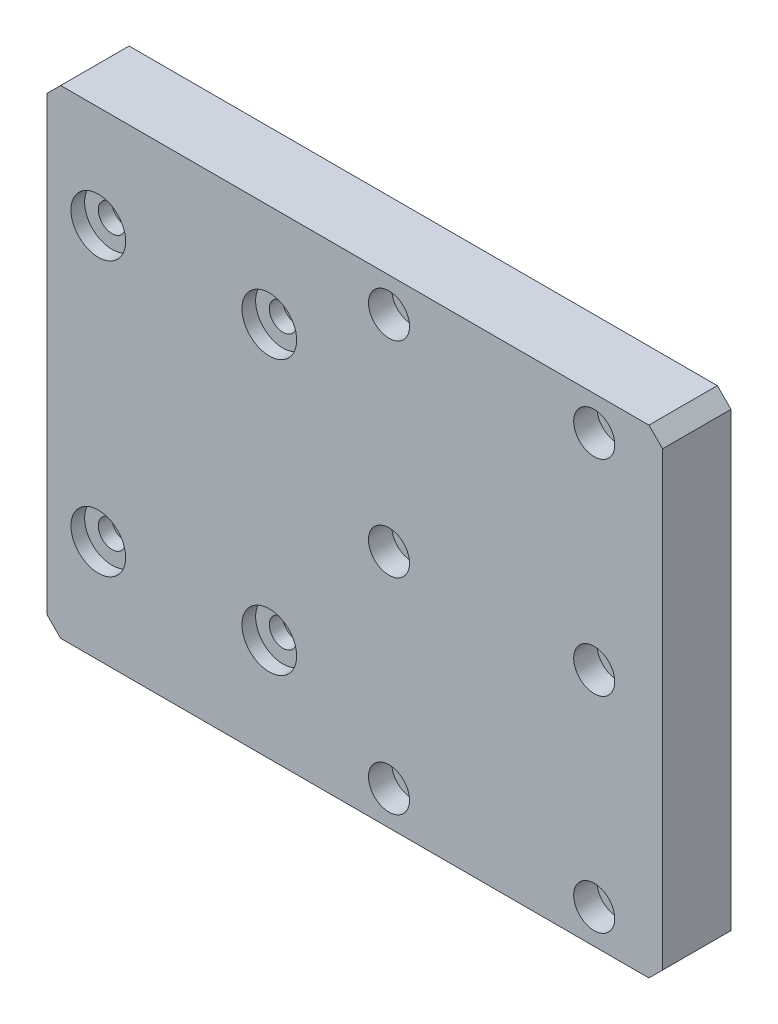
from build123d import *

# Parameters (mm, degrees)
SKETCH_1_W                = 90
SKETCH_1_H                = 70
EXTRUDE_1_DEPTH           = 5
HOLE_WIZARD_1_D           = 3.4
HOLE_WIZARD_1_CBORE_D     = 6
HOLE_WIZARD_1_CBORE_DEPTH = 3.4
HOLE_WIZARD_3_D           = 3.2
HOLE_WIZARD_3_CBORE_D     = 6
HOLE_WIZARD_3_CBORE_DEPTH = 3.4
SKETCH_6_R                = 4
CUT_EXTRUDE_1_DEPTH       = 2
SKETCH_8_R                = 2
CUT_EXTRUDE_2_DEPTH       = 2
CHAMFER_1_SIZE            = 2


with BuildPart() as part:
    # 草图1 → 凸台-拉伸1 (new, symmetric)
    with BuildSketch(Plane.XY):
        Rectangle(SKETCH_1_W, SKETCH_1_H)
    extrude(amount=EXTRUDE_1_DEPTH, both=True)

    # 打孔尺寸(%根据)内六角圆柱头螺钉的类型1 (through all)
    with Locations(Plane.XY.offset(5)):
        with Locations((5, 30), (5, 0), (5, -30), (35, 30), (35, 0), (35, -30)):
            CounterBoreHole(HOLE_WIZARD_1_D / 2, HOLE_WIZARD_1_CBORE_D / 2, HOLE_WIZARD_1_CBORE_DEPTH)

    # 打孔尺寸(%根据)内六角圆柱头螺钉的类型3 (through all)
    with Locations(Plane(origin=(0, 0, -5), x_dir=(-1, 0, 0), z_dir=(0, 0, -1))):
        with Locations((37.5, 20), (12.5, 20), (12.5, -20), (37.5, -20)):
            CounterBoreHole(HOLE_WIZARD_3_D / 2, HOLE_WIZARD_3_CBORE_D / 2, HOLE_WIZARD_3_CBORE_DEPTH)

    # 草图6 → 切除-拉伸1 (cut)
    with BuildSketch(Plane.XY.offset(5)):
        with Locations((-37.5, 20)):
            Circle(SKETCH_6_R)
        with Locations((-12.5, 20)):
            Circle(SKETCH_6_R)
        with Locations((-37.5, -20)):
            Circle(SKETCH_6_R)
        with Locations((-12.5, -20)):
            Circle(SKETCH_6_R)
    extrude(amount=-CUT_EXTRUDE_1_DEPTH, mode=Mode.SUBTRACT)

    # 草图8 → 切除-拉伸2 (cut)
    with BuildSketch(Plane.XY.offset(3)):
        with Locations((-37.5, 20)):
            Circle(SKETCH_8_R)
        with Locations((-37.5, -20)):
            Circle(SKETCH_8_R)
        with Locations((-12.5, -20)):
            Circle(SKETCH_8_R)
        with Locations((-12.5, 20)):
            Circle(SKETCH_8_R)
    extrude(amount=-CUT_EXTRUDE_2_DEPTH, mode=Mode.SUBTRACT)

    # 倒角1
    chamfer_1_edges = [part.edges().sort_by_distance(p)[0] for p in [
        (45, -35, 0),
        (-45, -35, 0),
        (-45, 35, 0),
        (45, 35, 0),
    ]]
    chamfer(chamfer_1_edges, length=CHAMFER_1_SIZE)


solid = part.part
